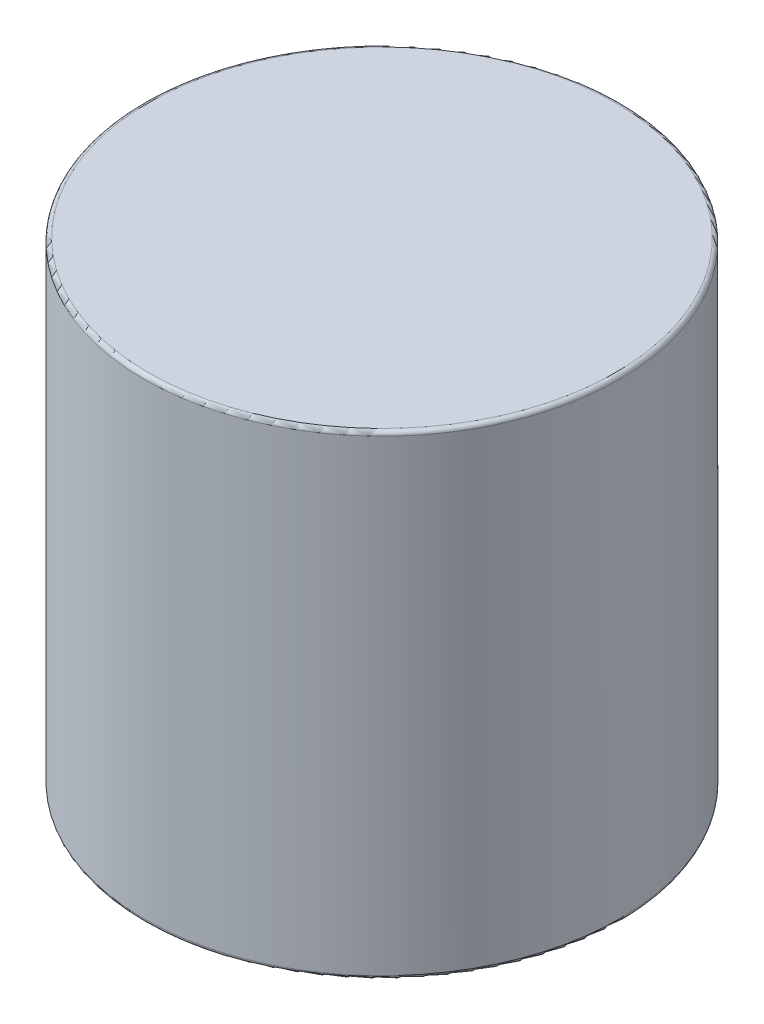
from build123d import *

# Parameters (mm, degrees)
SKETCH_1_W = 6
SKETCH_1_H = 12
FILLET_1_R = 0.1


with BuildPart() as part:
    # 草图1 → 旋转2 (revolve)
    with BuildSketch(Plane.XY, mode=Mode.PRIVATE) as revolve_2_sk:
        with Locations((3, 0)):
            Rectangle(SKETCH_1_W, SKETCH_1_H)
    revolve(revolve_2_sk.sketch.rotate(Axis((0, 6, 0), (0, -1, 0)), 90), axis=Axis((0, 6, 0), (0, -1, 0)))

    # 圆角1
    fillet_1_edges = [part.edges().sort_by_distance(p)[0] for p in [
        (0, -6, -6),
        (0, 6, -6),
    ]]
    fillet(fillet_1_edges, radius=FILLET_1_R)


solid = part.part
